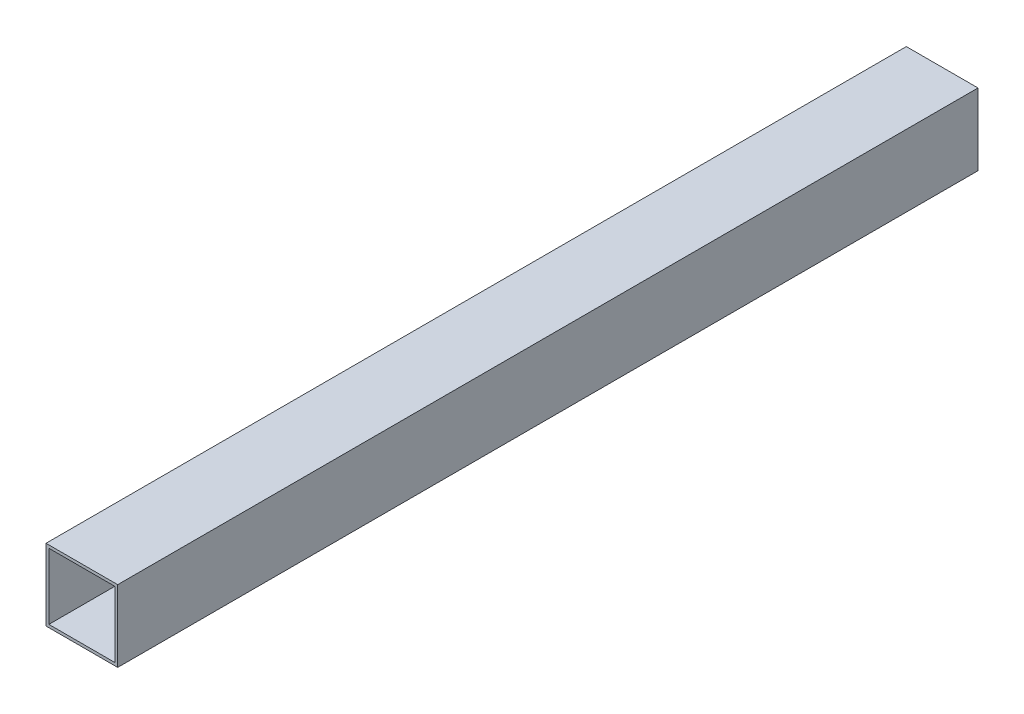
SolidWorks part; units mm, degrees
material "AISI 304"
ref_plane "Front Plane" through (0, 0, 0) normal (0, 0, 1) x (1, 0, 0)
ref_plane "Top Plane" through (0, 0, 0) normal (0, 1, 0) x (1, 0, 0)
ref_plane "Right Plane" through (0, 0, 0) normal (1, 0, 0) x (0, 0, -1)
sketch "Sketch1" plane through (0, 0, 0) normal (0, 0, 1) x (1, 0, 0)
  line L1 (-25, -25) -> (25, -25)
  line L2 (-25, -25) -> (-25, 25)
  line L3 (-25, 25) -> (25, 25)
  line L4 (25, -25) -> (25, 25)
  line L5 (-25, -25) -> (25, 25) construction
  line L6 (-25, 25) -> (25, -25) construction
  line L7 (-23, -23) -> (23, -23)
  line L8 (-23, -23) -> (-23, 23)
  line L9 (-23, 23) -> (23, 23)
  line L10 (23, -23) -> (23, 23)
  line L11 (-23, -23) -> (23, 23) construction
  line L12 (-23, 23) -> (23, -23) construction
  point P0 (0, 0)
  point P6 (0, 0)
  dimension "D1" = 50
  dimension "D2" = 50
  dimension "D3" = 46
  dimension "D4" = 46
extrude "Boss-Extrude1" add sketch "Sketch1" along normal blind 600
